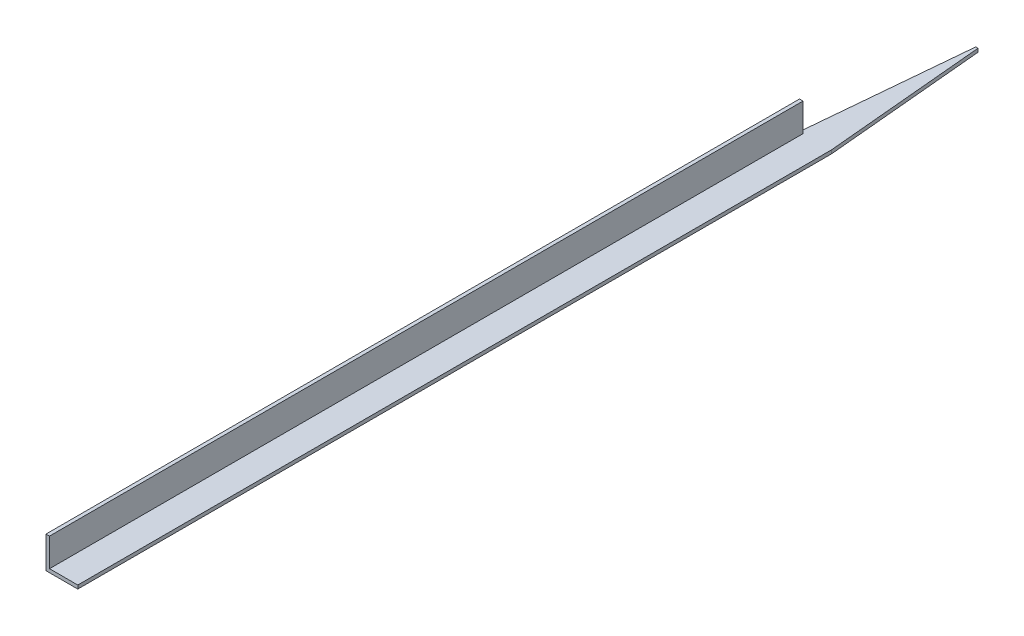
SolidWorks part; units mm, degrees
material "1023 碳钢板 (SS)"
ref_plane "Front Plane" through (0, 0, 0) normal (0, 0, 1) x (1, 0, 0)
ref_plane "Top Plane" through (0, 0, 0) normal (0, 1, 0) x (1, 0, 0)
ref_plane "Right Plane" through (0, 0, 0) normal (1, 0, 0) x (0, 0, -1)
sketch "Sketch1" plane through (0, 0, 0) normal (0, 0, 1) x (1, 0, 0)
  line L0 (-11.0054, 1.1403) -> (-11.0054, -43.8597)
  line L1 (-11.0054, -43.8597) -> (33.9946, -43.8597)
  line L2 (33.9946, -43.8597) -> (33.9946, -38.8597)
  line L3 (33.9946, -38.8597) -> (-6.0054, -38.8597)
  line L4 (-6.0054, -38.8597) -> (-6.0054, 1.1403)
  line L5 (-6.0054, 1.1403) -> (-11.0054, 1.1403)
  dimension "D1" = 5
  dimension "D2" = 5
  dimension "D3" = 45
  dimension "D4" = 45
extrude "Extrude1" add sketch "Sketch1" along normal blind 1295.4
ref_plane "Plane1" through (-6.0054, 1.1403, 0) normal (0, 1, 0) x (-1, 0, 0)
sketch "Sketch2" plane through (0, -43.8597, 0) normal (0, -1, 0) x (1, 0, 0)
  line L0 (-11.0054, 0) -> (33.9946, 0) construction
  line L1 (-11.0054, 0) -> (9.9046, 0)
  line L2 (11.4946, 1295.4) -> (11.4946, 0) construction
  line L3 (-11.0054, 1295.4) -> (-11.0054, 0) construction
  line L5 (-11.0054, 1295.4) -> (33.9946, 1295.4) construction
  line L6 (-11.0054, 228.6) -> (-11.0054, 0)
  line L7 (-11.0054, 228.6) -> (9.9046, 0)
  line L8 (-11.0054, 0) -> (33.9946, 0) construction
  line L9 (33.9946, 228.6) -> (13.0846, 0)
  line L10 (33.9946, 228.6) -> (33.9946, 0)
  line L11 (33.9946, 0) -> (13.0846, 0)
  dimension "D1" = 20.91
  dimension "D2" = 228.6
extrude "Extrude2" cut sketch "Sketch2" against normal through all
sketch "Sketch5" plane through (-6.0054, 0, 0) normal (1, 0, 0) x (0, 0, -1)
  line L0 (-173.9372, -38.8597) -> (-173.9372, 1.1403) construction
  line L1 (-173.9372, -38.8597) -> (-173.9372, 1.1403)
  line L2 (-173.9372, 1.1403) -> (-228.6, 1.1403)
  line L3 (-1295.4, 1.1403) -> (-173.9372, 1.1403) construction
  line L4 (-228.6, 1.1403) -> (-228.6, -38.8597)
  line L5 (-1295.4, -38.8597) -> (-173.9372, -38.8597) construction
  line L6 (-228.6, -38.8597) -> (-173.9372, -38.8597)
  line L8 (-1295.4, 1.1403) -> (-173.9372, 1.1403) construction
  line L9 (55, 1.1403) -> (-55, 1.1403) construction
extrude "Extrude3" cut sketch "Sketch5" against normal through all
